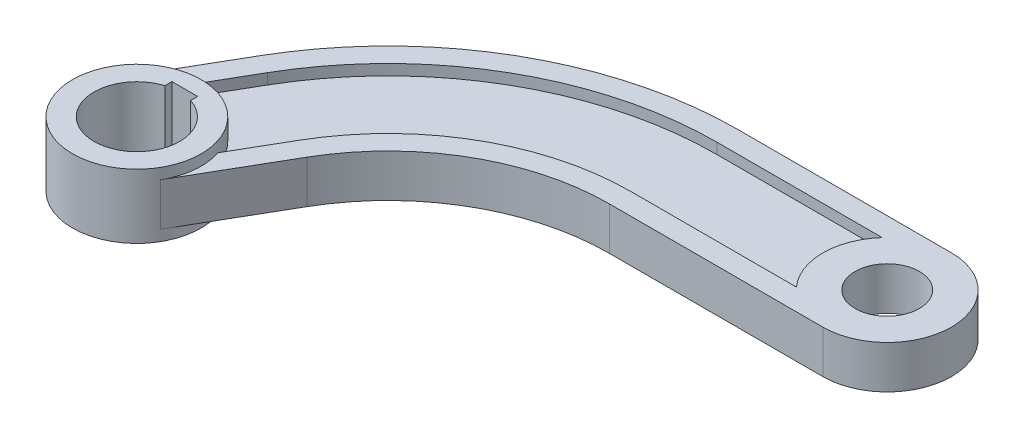
SolidWorks part; units mm, degrees
ref_plane "前视基准面" through (0, 0, 0) normal (0, 0, 1) x (1, 0, 0)
ref_plane "上视基准面" through (0, 0, 0) normal (0, 1, 0) x (1, 0, 0)
ref_plane "右视基准面" through (0, 0, 0) normal (1, 0, 0) x (0, 0, -1)
sketch "草图1" plane through (0, 0, 0) normal (0, 1, 0) x (1, 0, 0)
  line L0 (0, 24.816) -> (0, -14.1376) construction
  line L2 (6, 19.0788) -> (6, 22.3788)
  line L3 (6, 22.3788) -> (-6, 22.3788)
  line L4 (-6, 22.3788) -> (-6, 19.0788)
  circle A0 centre (0, 0) radius 30
  arc A1 (-6, 19.0788) -> (6, 19.0788) centre (0, 0) ccw
  dimension "D1" = 3.3
extrude "凸台-拉伸1" add sketch "草图1" along normal mid plane 30
sketch "草图2" plane through (0, 0, 0) normal (0, 1, 0) x (1, 0, 0)
  line L0 (-25.9808, 15) -> (-0.9808, 58.3013)
  line L1 (240, 80) -> (140.5256, 80)
  line L2 (50.9808, 28.3013) -> (25.9808, -15)
  line L6 (140.5256, 140) -> (240, 140)
  circle A0 centre (0, 0) radius 30 construction
  arc A1 (-25.9808, 15) -> (25.9808, -15) centre (0, 0) cw
  arc A2 (50.9808, 28.3013) -> (140.5256, 80) centre (140.5256, -23.3975) cw
  arc A3 (-0.9808, 58.3013) -> (140.5256, 140) centre (140.5256, -23.3975) cw
  arc A5 (240, 80) -> (240, 140) centre (240, 110) ccw
  circle A6 centre (240, 110) radius 15
  dimension "D1" = 50
extrude "凸台-拉伸2" add sketch "草图2" along normal mid plane 20
sketch "草图3" plane through (0, 0, 0) normal (0, 1, 0) x (1, 0, 0)
  circle A0 centre (240, 110) radius 15
  circle A1 centre (240, 110) radius 30
extrude "凸台-拉伸3" add sketch "草图3" along normal mid plane 20
sketch "草图4" plane through (0, 10, 0) normal (0, 1, 0) x (1, 0, 0)
  line L1 (217.6393, 130) -> (140.5256, 130)
  line L2 (140.5256, 90) -> (217.6393, 90)
  line L5 (28.5008, 9.3649) -> (42.3205, 33.3013)
  line L10 (7.6795, 53.3013) -> (-6.1402, 29.3649)
  arc A8 (217.6393, 130) -> (217.6393, 90) centre (240, 110) ccw
  arc A9 (28.5008, 9.3649) -> (-6.1402, 29.3649) centre (0, 0) ccw
  arc A10 (140.5256, 90) -> (42.3205, 33.3013) centre (140.5256, -23.3975) ccw
  arc A14 (140.5256, 130) -> (7.6795, 53.3013) centre (140.5256, -23.3975) ccw
extrude "切除-拉伸1" cut sketch "草图4" against normal blind 5
sketch "草图5" plane through (0, -10, 0) normal (0, -1, 0) x (1, 0, 0)
  line L0 (217.6393, -90) -> (140.5256, -90)
  line L1 (217.6393, -130) -> (140.5256, -130)
  line L2 (28.5008, -9.3649) -> (42.3205, -33.3013)
  line L3 (-6.1402, -29.3649) -> (7.6795, -53.3013)
  arc A1 (-6.1402, -29.3649) -> (28.5008, -9.3649) centre (0, 0) ccw
  arc A2 (7.6795, -53.3013) -> (140.5256, -130) centre (140.5256, 23.3975) ccw
  arc A3 (140.5256, -90) -> (42.3205, -33.3013) centre (140.5256, 23.3975) cw
  arc A5 (217.6393, -90) -> (217.6393, -130) centre (240, -110) ccw
extrude "切除-拉伸2" cut sketch "草图5" against normal blind 5
